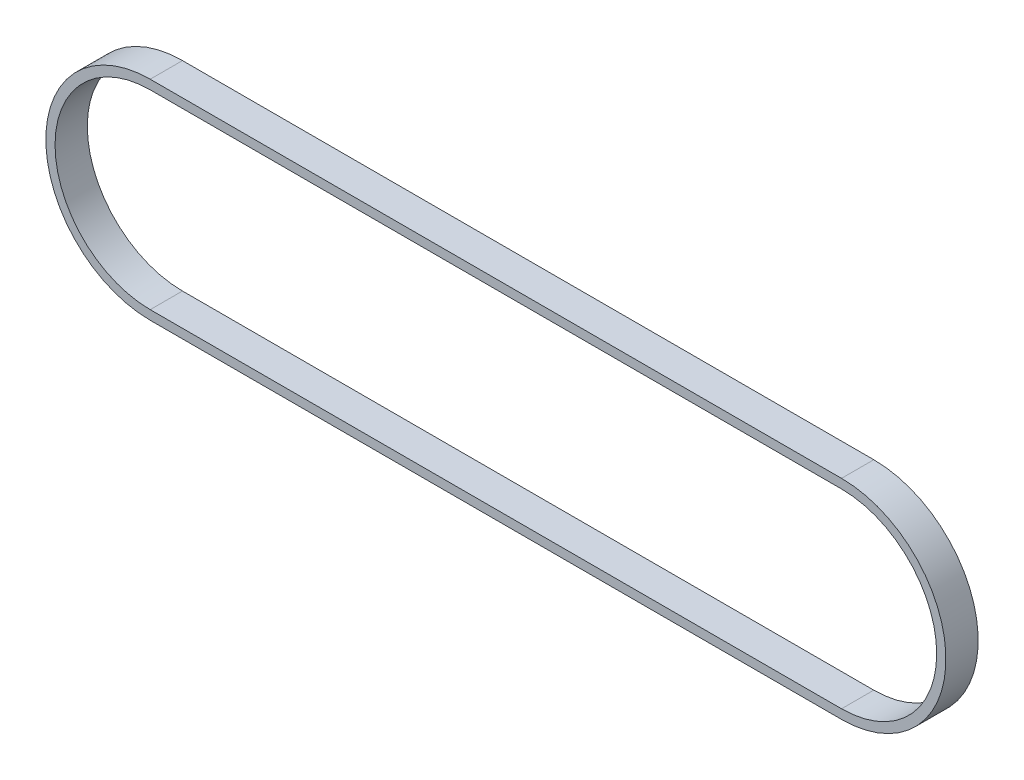
SolidWorks part; units mm, degrees
ref_plane "前视基准面" through (0, 0, 0) normal (0, 0, 1) x (1, 0, 0)
ref_plane "上视基准面" through (0, 0, 0) normal (0, 1, 0) x (1, 0, 0)
ref_plane "右视基准面" through (0, 0, 0) normal (1, 0, 0) x (0, 0, -1)
sketch "草图1" plane through (0, 0, 0) normal (0, 0, 1) x (1, 0, 0)
  line L0 (0, 0) -> (150, 0) construction
  line L1 (0, 21.65) -> (150, 21.65)
  line L2 (0, -21.65) -> (150, -21.65)
  arc A0 (0, 21.65) -> (0, -21.65) centre (0, 0) ccw
  arc A1 (150, -21.65) -> (150, 21.65) centre (150, 0) ccw
  point P3 (75, 0)
  dimension "D2" = 21.65
  dimension "D1" = 150
extrude "拉伸-薄壁1" add sketch "草图1" along normal mid plane 7 thin thin type mid plane wall 2
